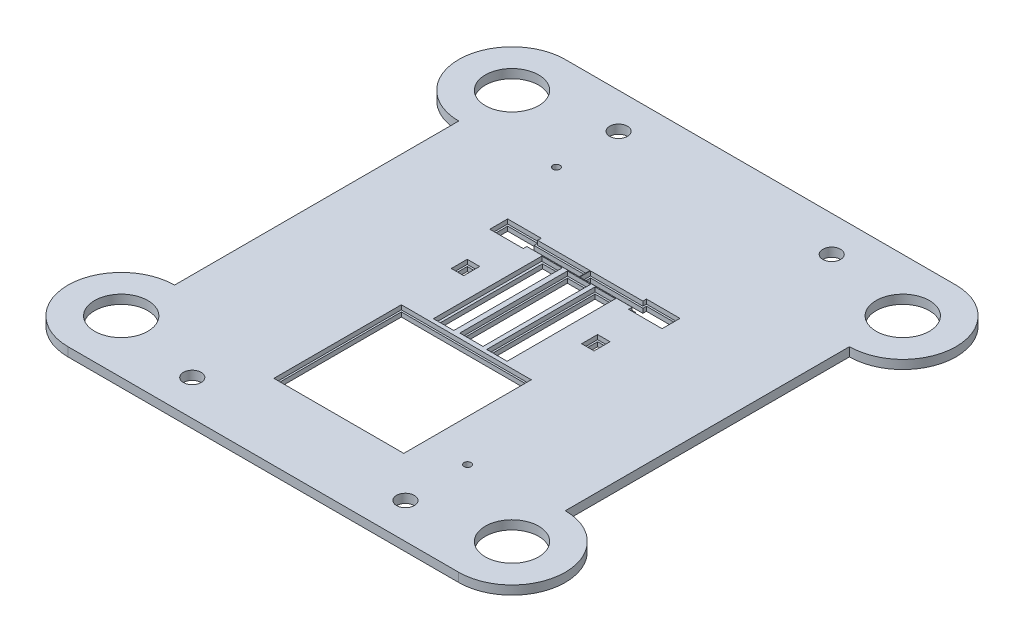
SolidWorks part; units mm, degrees
ref_plane "Front Plane" through (0, 0, 0) normal (0, 0, 1) x (1, 0, 0)
ref_plane "Top Plane" through (0, 0, 0) normal (0, 1, 0) x (1, 0, 0)
ref_plane "Right Plane" through (0, 0, 0) normal (1, 0, 0) x (0, 0, -1)
sketch "Sketch2" plane through (0, 0, 0) normal (0, 1, 0) x (1, 0, 0)
  line L0 (-80, -140) -> (110, -140)
  line L1 (110, -140) -> (110, 140)
  line L2 (110, 140) -> (-80, 140)
  line L3 (-80, -80) -> (-80, 80)
  arc A0 (-80, 140) -> (-80, 80) centre (-80, 110) ccw
  arc A1 (-80, -80) -> (-80, -140) centre (-80, -110) ccw
  circle A2 centre (-80, 110) radius 15
  circle A3 centre (-80, -110) radius 15
  dimension "D1" = 60
  dimension "D2" = 60
extrude "Boss-Extrude1" add sketch "Sketch2" along normal blind 5
sketch "Sketch3" plane through (0, 5, 0) normal (0, 1, 0) x (1, 0, 0)
  line L0 (0.37, 46.06) -> (0.37, 44.06)
  line L1 (-6.5722, -25.72) -> (66.5722, -25.72)
  line L2 (-6.5722, -25.72) -> (-6.5722, -97.5)
  line L3 (-6.5722, -97.5) -> (66.5722, -97.5)
  line L4 (66.5722, -25.72) -> (66.5722, -97.5)
  line L5 (-10.19, 15) -> (-3.19, 15)
  line L6 (-10.19, 15) -> (-10.19, 6)
  line L7 (-10.19, 6) -> (-3.19, 6)
  line L8 (-3.19, 15) -> (-3.19, 6)
  line L9 (63.19, 15) -> (70.19, 15)
  line L10 (63.19, 15) -> (63.19, 6)
  line L11 (63.19, 6) -> (70.19, 6)
  line L12 (70.19, 15) -> (70.19, 6)
  line L13 (39.25, 37.5) -> (50.75, 37.5)
  line L14 (39.25, 37.5) -> (39.25, -23.5)
  line L15 (39.25, -23.5) -> (50.75, -23.5)
  line L16 (50.75, 37.5) -> (50.75, -23.5)
  line L17 (23.69, 37.5) -> (36.75, 37.5)
  line L18 (23.69, 37.5) -> (23.69, -23.06)
  line L19 (23.69, -23.06) -> (36.75, -23.06)
  line L20 (36.75, 37.5) -> (36.75, -23.06)
  line L21 (9.25, 37.5) -> (20.75, 37.5)
  line L22 (9.25, 37.5) -> (9.25, -23.5)
  line L23 (9.25, -23.5) -> (20.75, -23.5)
  line L24 (20.75, 37.5) -> (20.75, -23.5)
  line L25 (-18.5, 46.06) -> (0.37, 46.06)
  line L26 (-18.5, 46.06) -> (-18.5, 36)
  line L27 (-18.5, 36) -> (0.37, 36)
  line L28 (29.86, 44.06) -> (29.86, 38)
  line L29 (78.5, 46.06) -> (59.63, 46.06)
  line L30 (78.5, 46.06) -> (78.5, 36)
  line L31 (78.5, 36) -> (59.63, 36)
  line L32 (30.14, 44.06) -> (30.14, 38)
  line L33 (0.37, 38) -> (29.86, 38)
  line L34 (0.37, 44.06) -> (29.86, 44.06)
  line L35 (30.14, 44.06) -> (59.63, 44.06)
  line L36 (30.14, 38) -> (59.63, 38)
  line L37 (59.63, 46.06) -> (59.63, 44.06)
  line L38 (59.63, 38) -> (59.63, 36)
  line L39 (0.37, 38) -> (0.37, 36)
extrude "Cut-Extrude1" cut sketch "Sketch3" against normal blind 2.5
sketch "Sketch4" plane through (0, 5, 0) normal (0, 1, 0) x (1, 0, 0)
  line L1 (24.69, 36.5) -> (35.75, 36.5)
  line L2 (35.75, 36.5) -> (35.75, -22.06)
  line L3 (24.69, -22.06) -> (35.75, -22.06)
  line L4 (24.69, 36.5) -> (24.69, -22.06)
  line L5 (30.0142, 36.5) -> (30.0142, 20.5985) construction
  line L6 (-0.6016, 45.06) -> (-0.6016, 43.06)
  line L7 (-17.4716, 45.06) -> (-17.4716, 37)
  line L8 (28.8884, 39) -> (-0.6016, 39)
  line L9 (-0.6016, 43.06) -> (28.8884, 43.06)
  line L10 (-0.6016, 45.06) -> (-17.4716, 45.06)
  line L11 (-0.6016, 37) -> (-17.4716, 37)
  line L12 (-0.6016, 39) -> (-0.6016, 37)
  line L13 (31.14, 43.06) -> (31.14, 39)
  line L14 (31.14, 39) -> (60.63, 39)
  line L15 (60.63, 39) -> (60.63, 37)
  line L16 (60.63, 37) -> (77.5, 37)
  line L18 (49.3384, 36.5) -> (49.3384, -22.5)
  line L19 (40.25, -22.5) -> (49.3384, -22.5)
  line L20 (40.25, 36.5) -> (40.25, -22.5)
  line L22 (64.19, 14) -> (69.19, 14)
  line L23 (60.63, 45.06) -> (77.5, 45.06)
  line L24 (77.5, 45.06) -> (77.5, 37)
  line L25 (60.63, 45.06) -> (60.63, 43.06)
  line L26 (60.63, 43.06) -> (31.14, 43.06)
  line L27 (69.19, 14) -> (69.19, 7)
  line L28 (64.19, 7) -> (69.19, 7)
  line L29 (64.19, 14) -> (64.19, 7)
  line L30 (-5.5722, -26.72) -> (65.5722, -26.72)
  line L31 (65.5722, -26.72) -> (65.5722, -96.5)
  line L32 (-5.5722, -96.5) -> (65.5722, -96.5)
  line L33 (-5.5722, -26.72) -> (-5.5722, -96.5)
  line L34 (28.8884, 43.06) -> (28.8884, 39)
  line L35 (19.7784, 36.5) -> (19.7784, -22.5)
  line L36 (19.7784, -22.5) -> (10.69, -22.5)
  line L37 (10.69, 36.5) -> (10.69, -22.5)
  line L38 (49.3384, 36.5) -> (40.25, 36.5)
  line L39 (-4.1616, 14) -> (-4.1616, 7)
  line L40 (-4.1616, 7) -> (-9.1616, 7)
  line L41 (-9.1616, 14) -> (-9.1616, 7)
  line L42 (-4.1616, 14) -> (-9.1616, 14)
  line L43 (10.69, 36.5) -> (19.7784, 36.5)
  dimension "D1" = 5
  dimension "D2" = 7
  dimension "D3" = 11.06
  dimension "D4" = 58.56
  dimension "D5" = 59
  dimension "D7" = 7
  dimension "D8" = 5
  dimension "D12" = 29.49
  dimension "D13" = 4.06
  dimension "D14" = 29.49
  dimension "D15" = 2
  dimension "D16" = 2
  dimension "D17" = 29.49
  dimension "D18" = 4.06
  dimension "D22" = 29.49
extrude "Cut-Extrude3" cut sketch "Sketch4" against normal blind 5
sketch "Sketch5" plane through (0, 5, 0) normal (0, 1, 0) x (1, 0, 0)
  circle A0 centre (-30, 120) radius 5
  circle A1 centre (90, 120) radius 5
  circle A2 centre (90, -120) radius 5
  circle A3 centre (-30, -120) radius 5
  dimension "D1" = 10
extrude "Cut-Extrude4" cut sketch "Sketch5" against normal through all
sketch "Sketch1" plane through (0, 5, 0) normal (0, 1, 0) x (1, 0, 0)
  line L0 (-30, 120) -> (90, -120) construction
  line L1 (-30, -120) -> (90, 120) construction
  line L2 (30, 0) -> (30, 244.9469) construction
  line L5 (108.0245, 140) -> (140, 140)
  line L6 (108.0245, 140) -> (108.0245, -140)
  line L7 (-80, 80) -> (-80, -80)
  line L8 (-80, -140) -> (110, -140)
  line L9 (110, -140) -> (110, 140)
  line L10 (110, 140) -> (-80, 140)
  line L12 (-80, -140) -> (-48.0245, -140)
  line L15 (140, -140) -> (108.0245, -140)
  line L16 (140, 80) -> (140, -80)
  arc A0 (140, -80) -> (140, -140) centre (140, -110) cw
  arc A1 (140, 140) -> (140, 80) centre (140, 110) cw
  arc A2 (-80, 140) -> (-80, 80) centre (-80, 110) ccw
  arc A3 (-80, -80) -> (-80, -140) centre (-80, -110) ccw
  arc A5 (-80, -80) -> (-80, -140) centre (-80, -110) ccw
  circle A6 centre (-80, -110) radius 15 construction
  circle A7 centre (-80, 110) radius 15 construction
  circle A8 centre (-80, -110) radius 15
  circle A9 centre (-80, 110) radius 15
  dimension "D1" = 0
extrude "Boss-Extrude2" add sketch "Sketch1" against normal blind 5 contours L6 L15 A0 L16 A1 L5
sketch "草图2" plane through (0, 5, 0) normal (0, 1, 0) x (1, 0, 0)
  circle A0 centre (140, 110) radius 15
  circle A1 centre (140, -110) radius 15
  dimension "D2" = 30
  dimension "D3" = 30
extrude "Cut-Extrude2" cut sketch "草图2" against normal blind 5
sketch "草图3" plane through (0, 5, 0) normal (0, 1, 0) x (1, 0, 0)
  line L0 (-30, 120) -> (-30, -120) construction
  line L1 (90, 120) -> (90, -120) construction
  circle A0 centre (-30, 85) radius 2
  circle A1 centre (90, -85) radius 2
  dimension "D1" = 4
  dimension "D2" = 4
  dimension "D3" = 35
  dimension "D4" = 35
extrude "切除-拉伸3" cut sketch "草图3" against normal through all
